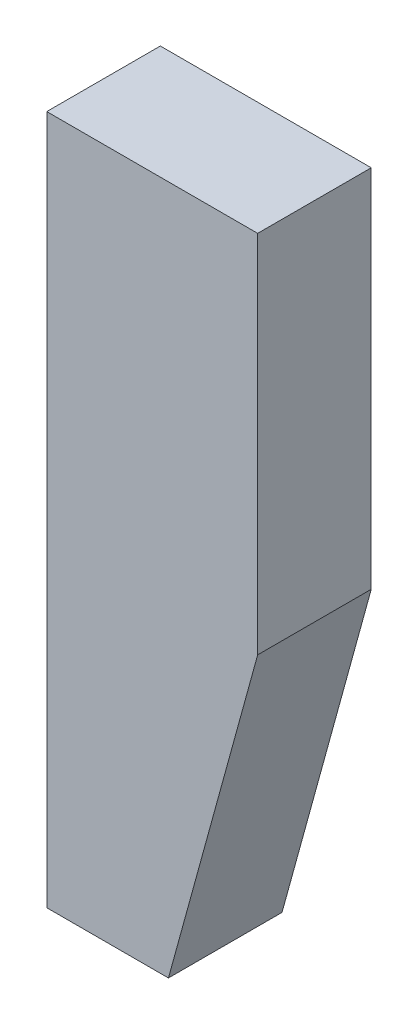
SolidWorks part; units mm, degrees
material "普通碳钢"
ref_plane "前视" through (0, 0, 0) normal (0, 0, 1) x (1, 0, 0)
ref_plane "上视" through (0, 0, 0) normal (0, 1, 0) x (1, 0, 0)
ref_plane "右视" through (0, 0, 0) normal (1, 0, 0) x (0, 0, -1)
sketch "草图1" plane through (0, 0, 0) normal (0, 0, 1) x (1, 0, 0)
  line L0 (-51.7568, 0) -> (56.6216, 0) construction
  line L1 (0, 105.971) -> (0, -40.2027) construction
  line L2 (0, 0) -> (0, 85)
  line L3 (0, 85) -> (26, 85)
  line L4 (26, 40) -> (26, 85)
  line L5 (26, 40) -> (15, 0)
  line L6 (15, 0) -> (0, 0)
  dimension "D1" = 26
  dimension "D2" = 85
  dimension "D3" = 45
  dimension "D4" = 15
extrude "凸台-拉伸1" add sketch "草图1" along normal mid plane 14
